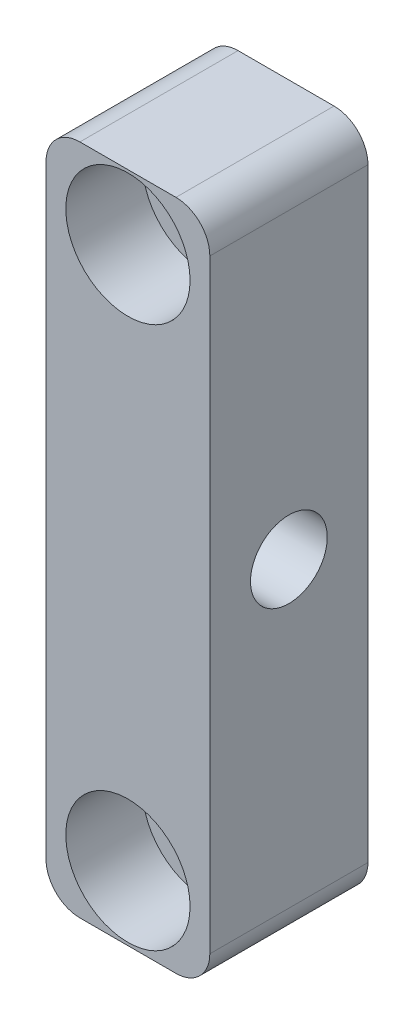
SolidWorks part; units mm, degrees
ref_plane "前视基准面" through (0, 0, 0) normal (0, 0, 1) x (1, 0, 0)
ref_plane "上视基准面" through (0, 0, 0) normal (0, 1, 0) x (1, 0, 0)
ref_plane "右视基准面" through (0, 0, 0) normal (1, 0, 0) x (0, 0, -1)
sketch "草图1" plane through (0, 0, 0) normal (0, 0, 1) x (1, 0, 0)
  line L1 (-7.25, 29.75) -> (7.25, 29.75)
  line L2 (-7.25, 29.75) -> (-7.25, -29.75)
  line L3 (-7.25, -29.75) -> (7.25, -29.75)
  line L4 (7.25, 29.75) -> (7.25, -29.75)
  line L5 (-7.25, 29.75) -> (7.25, -29.75) construction
  line L6 (-7.25, -29.75) -> (7.25, 29.75) construction
  point P0 (0, 0)
  dimension "D1" = 14.5
  dimension "D2" = 59.5
extrude "凸台-拉伸1" add sketch "草图1" along normal blind 14
fillet "圆角1" radius 3 4 edges at (7.25, 29.75, 7) (-7.25, 29.75, 7) (-7.25, -29.75, 7) (7.25, -29.75, 7)
hole_wizard "打孔尺寸(%根据)内六角圆柱头螺钉的类型2" positions "草图2" profile "草图3" counterbore size "M6" standard "GB" end condition through all
sketch "草图2" plane through (0, 0, 14) normal (0, 0, 1) x (1, 0, 0)
  line L0 (0, 0) -> (24.5678, 0) construction
  line L2 (0, 0) -> (0, 24) construction
  point P0 (0, 24)
  point P2 (0, -24)
  dimension "D1" = 48
sketch "草图3" plane through (0, 24, 14) normal (1, 0, 0) x (0, -1, 0)
  line L0 (0, 0) -> (0, 14)
  line L1 (0, 14) -> (3.3, 14)
  line L3 (3.3, 14) -> (3.3, 6.8)
  line L4 (3.3, 6.8) -> (5.5, 6.8)
  line L5 (5.5, 6.8) -> (5.5, 0)
  line L7 (5.5, 0) -> (0, 0)
  line L11 (0, -6.35) -> (0, 107.95) construction
  dimension "通孔孔直径" = 6.6
  dimension "通孔孔深度" = 14
  dimension "柱形沉头孔直径" = 11
  dimension "柱形沉头孔深度" = 6.8
hole_wizard "M8 螺纹孔1" positions "草图4" profile "草图5" tap size "M8" standard "GB" end condition through all
sketch "草图4" plane through (-7.25, 0, 0) normal (-1, 0, 0) x (0, 0, 1)
  line L0 (0, 0) -> (14, 0) construction
  line L1 (14, 26.75) -> (14, -26.75) construction
  point P0 (7, 0)
sketch "草图5" plane through (-7.25, 0, 7) normal (0, 1, 0) x (0, 0, 1)
  line L0 (0, 0) -> (0, 14.5)
  line L1 (0, 14.5) -> (3.4, 14.5)
  line L2 (3.4, 14.5) -> (3.4, 0)
  line L5 (3.4, 0) -> (0, 0)
  line L11 (0, -6.35) -> (0, 107.95) construction
  dimension "通孔螺纹孔钻头直径" = 6.8
  dimension "通孔螺纹孔钻头深度" = 14.5
cosmetic thread "孔螺蚊线3" parameters "D2"=8
